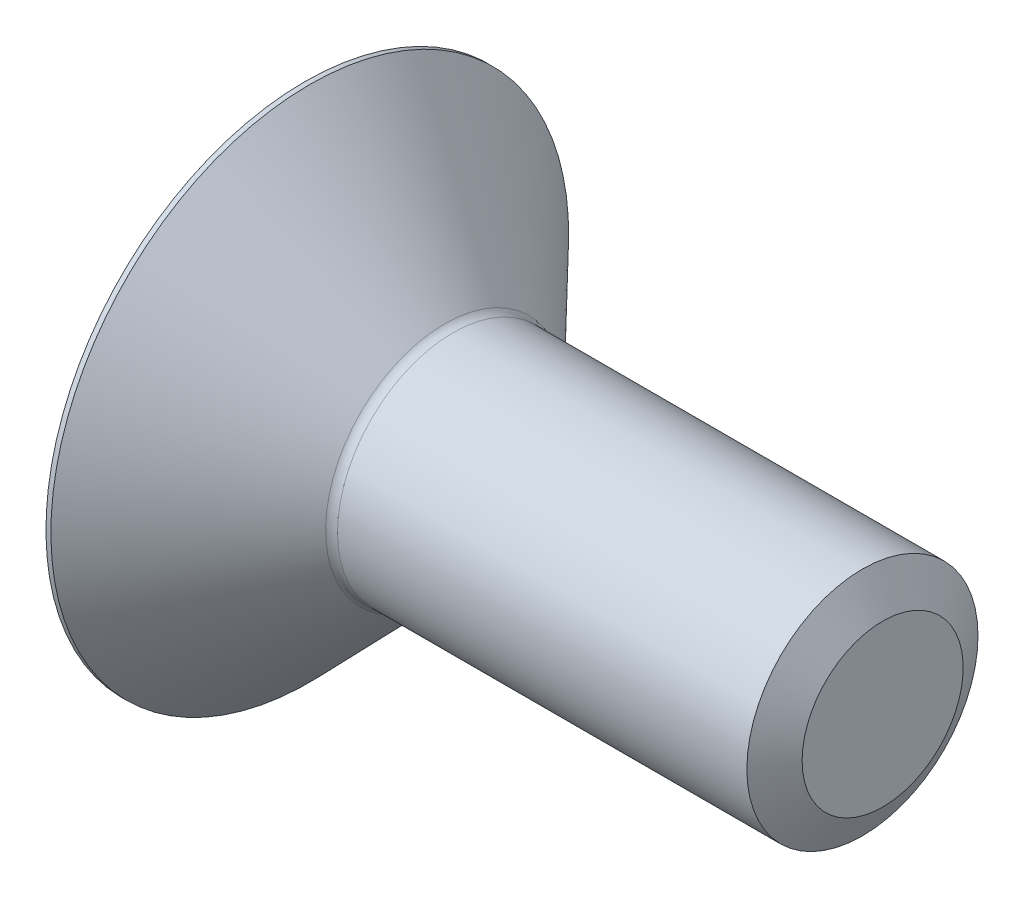
from build123d import *

# Parameters (mm, degrees)
CUT_EXTRUDE_1_DEPTH = 2.58


with BuildPart() as part:
    # 草图1 → 旋转1 (revolve)
    with BuildSketch(Plane.XY):
        with BuildLine():
            Line((0, 2), (-7.435105037, 2))
            ThreePointArc((-7.435105037, 2), (-7.513251262, 2.015899029), (-7.578972997, 2.061068326))
            Line((-7.578972997, 2.061068326), (-9.914908162, 4.48))
            Line((-9.914908162, 4.48), (-10, 4.48))
            Line((-10, 4.48), (-10, 0))
            Line((-10, 0), (0, 0))
            Line((0, 0), (0, 2))
        make_face()
    revolve(axis=Axis((0, 0, 0), (-1, 0, 0)))

    # 草图2 → 切除-拉伸1 (cut)
    with BuildSketch(Plane.ZY.offset(10)):
        Polygon((0, 1.443375673), (-1.25, 0.721687836), (-1.25, -0.721687836), (0, -1.443375673), (1.25, -0.721687836), (1.25, 0.721687836), align=None)
    extrude(amount=-CUT_EXTRUDE_1_DEPTH, mode=Mode.SUBTRACT)

    # 草图6 → 旋转2 (revolve)
    with BuildSketch(Plane.XY, mode=Mode.PRIVATE) as revolve_2_sk:
        Polygon((-8.5, 1.443375673), (-7.666666667, 0), (-7.05, 0), (-7.05, 1.443375673), align=None)
    revolve(revolve_2_sk.sketch.rotate(Axis((-10, 0, 0), (1, 0, 0)), 90), axis=Axis((-10, 0, 0), (1, 0, 0)))

    # 草图7 → 切除-旋转2 (revolve, cut)
    with BuildSketch(Plane.XY):
        Polygon((-10, 1.443375673), (-10, 0), (-9.593, 0), align=None)
    revolve(axis=Axis((-10, 0, 0), (1, 0, 0)), mode=Mode.SUBTRACT)

    # 草图4 → 切除-旋转1 (revolve, cut)
    with BuildSketch(Plane.XY):
        Polygon((-0.35, 2), (0, 1.393782217), (0.35, 2), align=None)
    revolve(axis=Axis((-0.35, 0, 0), (1, 0, 0)), mode=Mode.SUBTRACT)


solid = part.part
